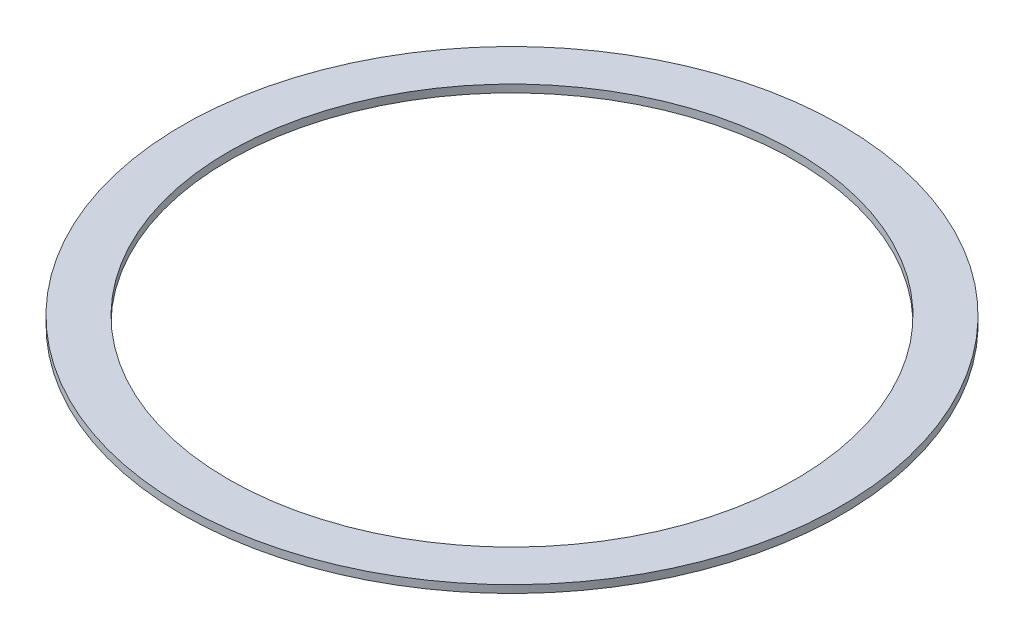
from build123d import *

# Parameters (mm, degrees)
SKETCH1_R           = 43
SKETCH1_R_2         = 37
BOSS_EXTRUDE1_DEPTH = 1


with BuildPart() as part:
    # Sketch1 → Boss-Extrude1 (new body)
    with BuildSketch(Plane(origin=(0, 0, 0), x_dir=(1, 0, 0), z_dir=(0, 1, 0))):
        with Locations(Location((0, 0, 0), (0, 0, 270))):
            Circle(SKETCH1_R)
        with Locations(Location((0, 0, 0), (0, 0, 270))):
            Circle(SKETCH1_R_2, mode=Mode.SUBTRACT)
    extrude(amount=BOSS_EXTRUDE1_DEPTH)


solid = part.part
